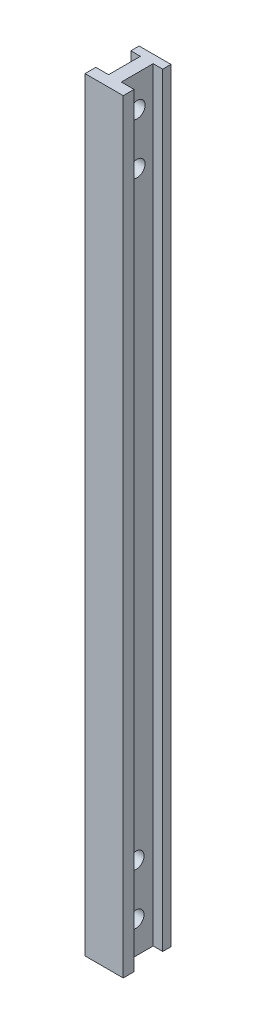
SolidWorks part; units mm, degrees
ref_plane "Front Plane" through (0, 0, 0) normal (0, 0, 1) x (1, 0, 0)
ref_plane "Top Plane" through (0, 0, 0) normal (0, 1, 0) x (1, 0, 0)
ref_plane "Right Plane" through (0, 0, 0) normal (1, 0, 0) x (0, 0, -1)
other "Configuration Table"
sketch "Sketch1" plane through (0, 0, 0) normal (0, 1, 0) x (1, 0, 0)
  line L0 (10, 27) -> (25, 27)
  line L2 (-10, 27) -> (-10, -23)
  line L4 (10, 27) -> (10, -23)
  line L5 (-10, 40) -> (10, -40) construction
  line L6 (-10, -40) -> (10, 40) construction
  line L7 (-25, 40) -> (25, 40)
  line L8 (-25, 40) -> (-25, 27)
  line L9 (-25, 27) -> (-10, 27)
  line L10 (25, 40) -> (25, 27)
  line L11 (30, -40) -> (-30, -40)
  line L12 (30, -40) -> (30, -23)
  line L13 (30, -23) -> (10, -23)
  line L14 (-30, -40) -> (-30, -23)
  line L15 (-10, -23) -> (-30, -23)
  point P0 (0, 0)
  dimension "D1" = 20
  dimension "D2" = 50
  dimension "D3" = 15
  dimension "D4" = 20
  dimension "D5" = 60
  dimension "D6" = 13
  dimension "D7" = 17
  dimension "D8" = 80
  dimension "D9" = 20
extrude "Boss-Extrude1" add sketch "Sketch1" along normal blind 1200
sketch "Sketch2" plane through (10, 0, 0) normal (1, 0, 0) x (0, 0, -1)
  line L0 (2, 1200) -> (0, 0) construction
  line L1 (-23, 1200) -> (27, 1200) construction
  line L2 (-23, 0) -> (27, 0) construction
  circle A0 centre (1.9167, 1150) radius 12.5
  circle A1 centre (1.7833, 1070) radius 12.5
  circle A2 centre (0.0833, 50) radius 12.5
  circle A3 centre (0.2167, 130) radius 12.5
  dimension "D1" = 25
  dimension "D2" = 25
  dimension "D5" = 25
  dimension "D6" = 25
  dimension "D3" = 50
  dimension "D4" = 80
  dimension "D7" = 80
  dimension "D8" = 50
extrude "Cut-Extrude1" cut sketch "Sketch2" against normal up to next
